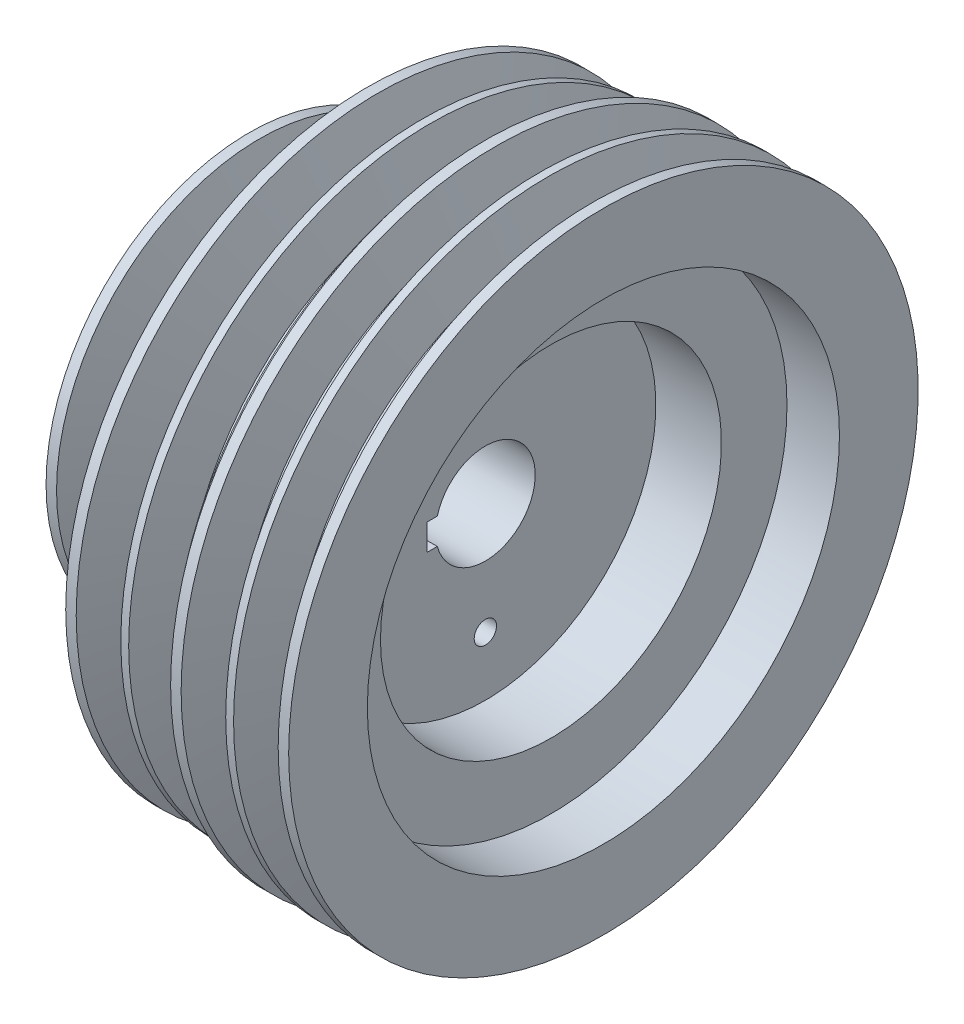
from build123d import *

# Parameters (mm, degrees)
CUT_EXTRUDE_1_REACH     = 194.094
SKETCH_2_W              = 3.96969722
SKETCH_2_H              = 10
HOLE_WIZARD_M10_2_D     = 8.5
HOLE_WIZARD_M10_2_DEPTH = 24.5
HOLE_WIZARD_M10_2_TIP   = 2.553657631


with BuildPart() as part:
    # 草图1 → 旋转1 (revolve)
    with BuildSketch(Plane.XY, mode=Mode.PRIVATE) as revolve_1_sk:
        Polygon((0, 77.5), (0, 19), (90, 19), (90, 65), (115, 65), (115, 90), (135, 90), (135, 120), (131, 120), (124.858175439, 104), (118.891690903, 104), (114, 120), (111, 120), (104.858175439, 104), (98.891690903, 104), (94, 120), (90, 120), (90, 115), (86, 115), (79.858175439, 99), (73.891690903, 99), (69, 115), (66, 115), (61.108309097, 99), (55.141824561, 99), (49, 115), (45, 115), (45, 77.5), (41, 77.5), (36.108309097, 61.5), (28.891690903, 61.5), (24, 77.5), (21, 77.5), (16.108309097, 61.5), (8.891690903, 61.5), (4, 77.5), align=None)
    revolve(revolve_1_sk.sketch.rotate(Axis((0, 0, 0), (1, 0, 0)), 90), axis=Axis((0, 0, 0), (1, 0, 0)))

    # 草图2 → 切除-拉伸1 (cut, up to next)
    with BuildSketch(Plane(origin=(90, 0, 0), x_dir=(0, 0, -1), z_dir=(1, 0, 0)), mode=Mode.PRIVATE) as cut_extrude_1_sk1:
        with Locations((-20.31515139, 0)):
            Rectangle(SKETCH_2_W, SKETCH_2_H)
    cut_extrude_1_tool1 = extrude(cut_extrude_1_sk1.sketch, amount=-CUT_EXTRUDE_1_REACH, mode=Mode.PRIVATE) & part.part
    add(cut_extrude_1_tool1.solids().sort_by_distance((90, 0, 20.315151))[0], mode=Mode.SUBTRACT)

    # M10 螺纹孔2
    with Locations(Plane(origin=(90, 0, 0), x_dir=(0, 0, -1), z_dir=(1, 0, 0))):
        with Locations((0, 42.5), (0, -42.5)):
            Hole(HOLE_WIZARD_M10_2_D / 2, depth=HOLE_WIZARD_M10_2_DEPTH)
            with Locations((0, 0, -(HOLE_WIZARD_M10_2_DEPTH + HOLE_WIZARD_M10_2_TIP / 2))):  # 118° drill point
                Cone(0, HOLE_WIZARD_M10_2_D / 2, HOLE_WIZARD_M10_2_TIP, mode=Mode.SUBTRACT)


solid = part.part
